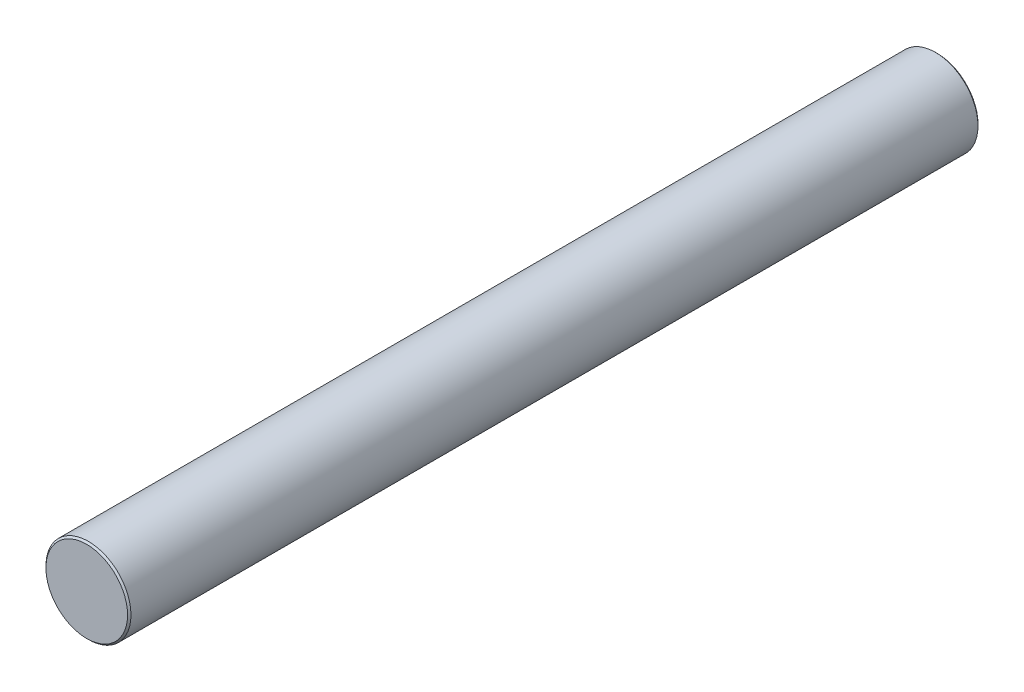
from build123d import *

# Parameters (mm, degrees)
SKETCH1_R           = 2.5
BOSS_EXTRUDE1_DEPTH = 25
CHAMFER1_SIZE       = 0.1


with BuildPart() as part:
    # Sketch1 → Boss-Extrude1 (new, symmetric)
    with BuildSketch(Plane.XY):
        Circle(SKETCH1_R)
    extrude(amount=BOSS_EXTRUDE1_DEPTH, both=True)

    # Chamfer1
    chamfer1_edges = [part.edges().sort_by_distance(p)[0] for p in [
        (-2.5, 0, -25),
        (-2.5, 0, 25),
    ]]
    chamfer(chamfer1_edges, length=CHAMFER1_SIZE)


solid = part.part
